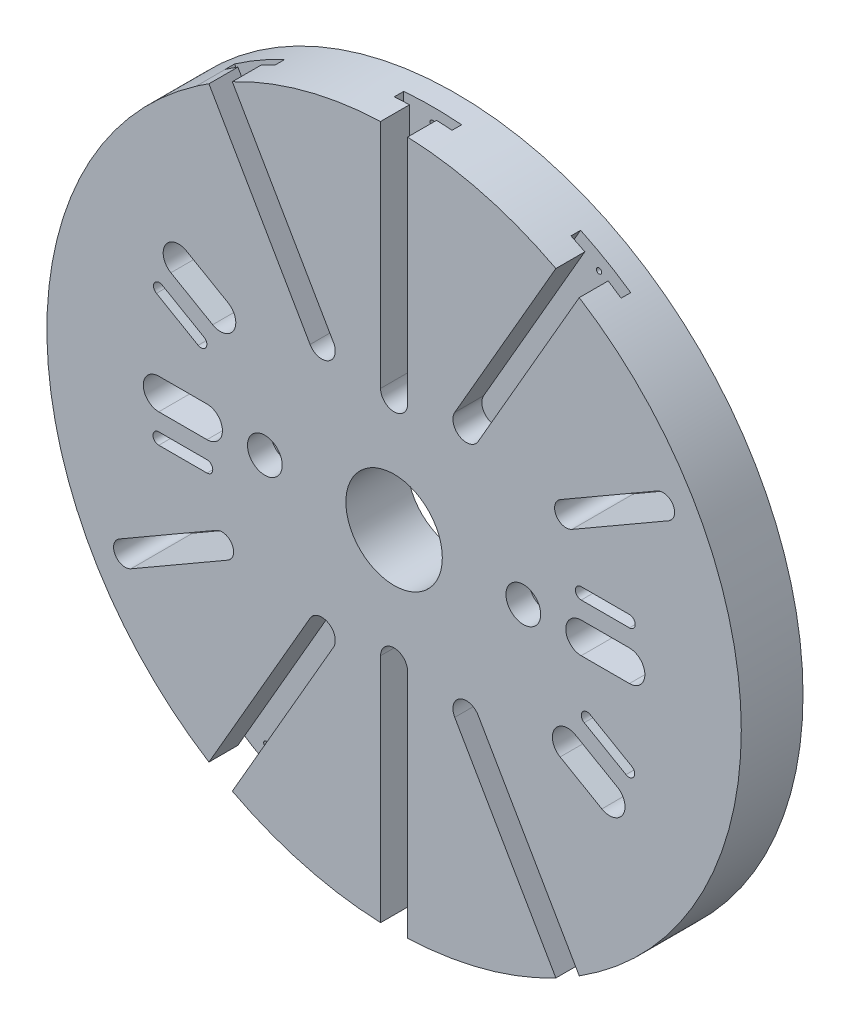
SolidWorks part; units mm, degrees
ref_plane "Front Plane" through (0, 0, 0) normal (0, 0, 1) x (1, 0, 0)
ref_plane "Top Plane" through (0, 0, 0) normal (0, 1, 0) x (1, 0, 0)
ref_plane "Right Plane" through (0, 0, 0) normal (1, 0, 0) x (0, 0, -1)
sketch "Sketch1" plane through (0, 0, 0) normal (0, 0, 1) x (1, 0, 0)
  circle A0 centre (0, 0) radius 180
  circle A1 centre (0, 0) radius 25
extrude "Boss-Extrude1" add sketch "Sketch1" along normal blind 32 contours A0 | A1
sketch "Sketch2" plane through (0, 0, 32) normal (0, 0, 1) x (1, 0, 0)
  line L0 (-198.9855, 0) -> (202.4357, 0) construction
  line L1 (0, 209.2415) -> (0, -209.2454) construction
  circle A0 centre (67, 0) radius 5.5
  circle A1 centre (-67, 0) radius 5.5
  dimension "D2" = 11
  dimension "D1" = 67
extrude "Cut-Extrude1" cut sketch "Sketch2" against normal through all
sketch "Sketch3" plane through (0, 0, 32) normal (0, 0, 1) x (1, 0, 0)
  line L1 (-86.2006, -56.6962) -> (-136.4301, -85.6962)
  line L3 (86.2006, 56.6962) -> (136.4301, 85.6962)
  line L4 (92.2006, 46.3038) -> (142.4301, 75.3038)
  line L5 (-92.2006, -46.3038) -> (-142.4301, -75.3038)
  arc A0 (86.2006, 56.6962) -> (92.2006, 46.3038) centre (89.2006, 51.5) ccw
  arc A1 (142.4301, 75.3038) -> (136.4301, 85.6962) centre (139.4301, 80.5) ccw
  arc A4 (-136.4301, -85.6962) -> (-142.4301, -75.3038) centre (-139.4301, -80.5) cw
  arc A5 (-92.2006, -46.3038) -> (-86.2006, -56.6962) centre (-89.2006, -51.5) cw
  dimension "D5" = 12
  dimension "D6" = 12
  dimension "D4" = 58
extrude "Cut-Extrude3" cut sketch "Sketch3" against normal through all contours L4 A1 L3 A0
ref_plane "Plane1" through (0, 0, 12) normal (0, 0, -1) x (-1, 0, 0)
sketch "Sketch5" plane through (0, 0, 12) normal (0, 0, -1) x (-1, 0, 0)
  line L1 (15, 60) -> (15, 264.0611)
  line L2 (-15, 60) -> (-15, 249.3757)
  line L3 (15, 264.0611) -> (-15, 249.3757)
  line L4 (-91.9564, 189.2731) -> (-117.9372, 174.2731)
  line L5 (-117.9372, 174.2731) -> (-50.4904, 57.4519)
  line L6 (-91.9564, 189.2731) -> (-24.5096, 72.4519)
  line L7 (91.9564, 189.2731) -> (24.5096, 72.4519)
  line L8 (117.9372, 174.2731) -> (50.4904, 57.4519)
  line L9 (91.9564, 189.2731) -> (117.9372, 174.2731)
  line L11 (91.9564, -189.2731) -> (117.9372, -174.2731)
  line L12 (117.9372, -174.2731) -> (50.4904, -57.4519)
  line L13 (91.9564, -189.2731) -> (24.5096, -72.4519)
  line L14 (-91.9564, -189.2731) -> (-24.5096, -72.4519)
  line L15 (-117.9372, -174.2731) -> (-50.4904, -57.4519)
  line L16 (-91.9564, -189.2731) -> (-117.9372, -174.2731)
  line L17 (10, -264.0611) -> (-15, -249.3757)
  line L18 (-15, -60) -> (-15, -249.3757)
  line L19 (15, -60) -> (10, -264.0611)
  arc A0 (-15, 60) -> (15, 60) centre (0, 60) ccw
  arc A2 (-50.4904, 57.4519) -> (-24.5096, 72.4519) centre (-37.5, 64.9519) ccw
  arc A3 (50.4904, 57.4519) -> (24.5096, 72.4519) centre (37.5, 64.9519) cw
  arc A4 (50.4904, -57.4519) -> (24.5096, -72.4519) centre (37.5, -64.9519) ccw
  arc A5 (-50.4904, -57.4519) -> (-24.5096, -72.4519) centre (-37.5, -64.9519) cw
  arc A6 (-15, -60) -> (15, -60) centre (0, -60) cw
  dimension "D1" = 15
  dimension "D3" = 15
  dimension "D4" = 15
  dimension "D2" = 15
  dimension "D5" = 15
  dimension "D6" = 15
extrude "Cut-Extrude4" cut sketch "Sketch5" against normal blind 5
sketch "Sketch6" plane through (0, 0, 32) normal (0, 0, 1) x (1, 0, 0)
  line L1 (-95.8846, -180.077) -> (-108.0089, -173.077)
  line L2 (-108.0089, -173.077) -> (-43.5622, -61.4519)
  line L3 (-31.4378, -68.4519) -> (-95.8846, -180.077)
  line L4 (-7, -254.4437) -> (-7, -60)
  line L5 (7, -245.6325) -> (-7, -254.4437)
  line L6 (7, -60) -> (7, -245.6325)
  line L7 (43.5622, -61.4519) -> (108.0089, -173.077)
  line L8 (95.8846, -180.077) -> (31.4378, -68.4519)
  line L9 (108.0089, 173.077) -> (95.8846, 180.077)
  line L10 (95.8846, 180.077) -> (31.4378, 68.4519)
  line L11 (43.5622, 61.4519) -> (108.0089, 173.077)
  line L12 (108.0089, -173.077) -> (95.8846, -180.077)
  line L18 (7, 60) -> (7, 245.6325)
  line L19 (7, 245.6325) -> (-7, 254.4437)
  line L20 (-7, 254.4437) -> (-7, 60)
  line L27 (-31.4378, 68.4519) -> (-95.8846, 180.077)
  line L28 (-108.0089, 173.077) -> (-43.5622, 61.4519)
  line L29 (-95.8846, 180.077) -> (-108.0089, 173.077)
  arc A0 (-43.5622, -61.4519) -> (-31.4378, -68.4519) centre (-37.5, -64.9519) cw
  arc A1 (-7, -60) -> (7, -60) centre (0, -60) cw
  arc A2 (31.4378, -68.4519) -> (43.5622, -61.4519) centre (37.5, -64.9519) cw
  arc A3 (31.4378, 68.4519) -> (43.5622, 61.4519) centre (37.5, 64.9519) ccw
  arc A6 (-7, 60) -> (7, 60) centre (0, 60) ccw
  arc A9 (-43.5622, 61.4519) -> (-31.4378, 68.4519) centre (-37.5, 64.9519) ccw
  dimension "D1" = 7
  dimension "D2" = 7
  dimension "D3" = 7
extrude "Cut-Extrude5" cut sketch "Sketch6" against normal up to next
sketch "Sketch7" plane through (0, 0, 32) normal (0, 0, 1) x (1, 0, 0)
  line L0 (0, 0) -> (0, 172.5) construction
  line L1 (0, 0) -> (86.25, 149.3894) construction
  circle A0 centre (0, 172.5) radius 1.375
  arc A1 (15, 179.3739) -> (-15, 179.3739) centre (0, 0) ccw construction
  circle A2 centre (86.25, 149.3894) radius 1.375
  circle A3 centre (149.3894, 86.25) radius 1.375 [skipped]
  circle A4 centre (172.5, 0) radius 1.375 [skipped]
  circle A5 centre (149.3894, -86.25) radius 1.375 [skipped]
  circle A6 centre (86.25, -149.3894) radius 1.375
  circle A7 centre (0, -172.5) radius 1.375
  circle A8 centre (-86.25, -149.3894) radius 1.375
  circle A9 centre (-149.3894, -86.25) radius 1.375 [skipped]
  circle A10 centre (-172.5, 0) radius 1.375 [skipped]
  circle A11 centre (-149.3894, 86.25) radius 1.375 [skipped]
  circle A12 centre (-86.25, 149.3894) radius 1.375
  point P2 (0, 180)
  dimension "D1" = 2.75
  dimension "D2" = 7.5
  dimension "D3" = 30
extrude "Cut-Extrude6" cut sketch "Sketch7" against normal through all
sketch "Sketch8" plane through (0, 0, 32) normal (0, 0, 1) x (1, 0, 0)
  line L0 (0, 0) -> (229.3619, 0) construction
  line L1 (97, 8) -> (122, 8)
  line L2 (97, -8) -> (122, -8)
  line L3 (97, 23) -> (122, 23)
  line L4 (0, 0) -> (181.224, -104.6297) construction
  line L5 (0, 0) -> (-183.3392, 105.8509) construction
  line L6 (120.2173, -49.7776) -> (98.5666, -37.2776)
  line L7 (122, 17) -> (97, 17)
  line L9 (41.5718, -88.0045) -> (54.0718, -109.6551) [skipped]
  line L10 (55.4282, -80.0045) -> (67.9282, -101.6551) [skipped]
  line L11 (75.7224, -97.1551) -> (63.2224, -75.5045) [skipped]
  line L12 (68.4186, -72.5045) -> (80.9186, -94.1551) [skipped]
  line L13 (-8, -97) -> (-8, -122) [skipped]
  line L14 (8, -97) -> (8, -122) [skipped]
  line L15 (17, -122) -> (17, -97) [skipped]
  line L16 (23, -97) -> (23, -122) [skipped]
  line L17 (-55.4282, -80.0045) -> (-67.9282, -101.6551) [skipped]
  line L18 (-41.5718, -88.0045) -> (-54.0718, -109.6551) [skipped]
  line L19 (-46.2776, -114.1551) -> (-33.7776, -92.5045) [skipped]
  line L20 (-28.5814, -95.5045) -> (-41.0814, -117.1551) [skipped]
  line L21 (-88.0045, -41.5718) -> (-109.6551, -54.0718) [skipped]
  line L22 (-80.0045, -55.4282) -> (-101.6551, -67.9282) [skipped]
  line L23 (-97.1551, -75.7224) -> (-75.5045, -63.2224) [skipped]
  line L24 (-72.5045, -68.4186) -> (-94.1551, -80.9186) [skipped]
  line L25 (-97, 8) -> (-122, 8)
  line L26 (-97, -8) -> (-122, -8)
  line L27 (-122, -17) -> (-97, -17)
  line L28 (-97, -23) -> (-122, -23)
  line L30 (86.0666, -58.9282) -> (107.7173, -71.4282)
  line L31 (94.0666, -45.0718) -> (115.7173, -57.5718)
  line L32 (101.5666, -32.0814) -> (123.2173, -44.5814)
  line L33 (-41.5718, 88.0045) -> (-54.0718, 109.6551) [skipped]
  line L34 (-55.4282, 80.0045) -> (-67.9282, 101.6551) [skipped]
  line L35 (-75.7224, 97.1551) -> (-63.2224, 75.5045) [skipped]
  line L36 (-68.4186, 72.5045) -> (-80.9186, 94.1551) [skipped]
  line L37 (8, 97) -> (8, 122) [skipped]
  line L38 (-8, 97) -> (-8, 122) [skipped]
  line L39 (-17, 122) -> (-17, 97) [skipped]
  line L40 (-23, 97) -> (-23, 122) [skipped]
  line L41 (55.4282, 80.0045) -> (67.9282, 101.6551) [skipped]
  line L42 (41.5718, 88.0045) -> (54.0718, 109.6551) [skipped]
  line L43 (46.2776, 114.1551) -> (33.7776, 92.5045) [skipped]
  line L44 (28.5814, 95.5045) -> (41.0814, 117.1551) [skipped]
  line L45 (88.0045, 41.5718) -> (109.6551, 54.0718) [skipped]
  line L46 (80.0045, 55.4282) -> (101.6551, 67.9282) [skipped]
  line L47 (97.1551, 75.7224) -> (75.5045, 63.2224) [skipped]
  line L48 (72.5045, 68.4186) -> (94.1551, 80.9186) [skipped]
  line L49 (-86.0666, 58.9282) -> (-107.7173, 71.4282)
  line L50 (-94.0666, 45.0718) -> (-115.7173, 57.5718)
  line L51 (-120.2173, 49.7776) -> (-98.5666, 37.2776)
  line L52 (-101.5666, 32.0814) -> (-123.2173, 44.5814)
  line L53 (-80.0045, 55.4282) -> (-101.6551, 67.9282) [skipped]
  line L54 (-88.0045, 41.5718) -> (-109.6551, 54.0718) [skipped]
  line L55 (-114.1551, 46.2776) -> (-92.5045, 33.7776) [skipped]
  line L56 (-95.5045, 28.5814) -> (-117.1551, 41.0814) [skipped]
  line L57 (80.0045, -55.4282) -> (101.6551, -67.9282) [skipped]
  line L58 (88.0045, -41.5718) -> (109.6551, -54.0718) [skipped]
  line L59 (114.1551, -46.2776) -> (92.5045, -33.7776) [skipped]
  line L60 (95.5045, -28.5814) -> (117.1551, -41.0814) [skipped]
  arc A0 (97, 8) -> (97, -8) centre (97, 0) ccw
  arc A1 (122, -8) -> (122, 8) centre (122, 0) ccw
  arc A4 (97, 23) -> (97, 17) centre (97, 20) ccw
  arc A5 (122, 17) -> (122, 23) centre (122, 20) ccw
  arc A6 (115.7173, -57.5718) -> (107.7173, -71.4282) centre (111.7173, -64.5) cw
  arc A7 (86.0666, -58.9282) -> (94.0666, -45.0718) centre (90.0666, -52) cw
  arc A8 (55.4282, -80.0045) -> (41.5718, -88.0045) centre (48.5, -84.0045) ccw [skipped]
  arc A9 (54.0718, -109.6551) -> (67.9282, -101.6551) centre (61, -105.6551) ccw [skipped]
  arc A10 (68.4186, -72.5045) -> (63.2224, -75.5045) centre (65.8205, -74.0045) ccw [skipped]
  arc A11 (75.7224, -97.1551) -> (80.9186, -94.1551) centre (78.3205, -95.6551) ccw [skipped]
  arc A12 (8, -97) -> (-8, -97) centre (0, -97) ccw [skipped]
  arc A13 (-8, -122) -> (8, -122) centre (0, -122) ccw [skipped]
  arc A14 (23, -97) -> (17, -97) centre (20, -97) ccw [skipped]
  arc A15 (17, -122) -> (23, -122) centre (20, -122) ccw [skipped]
  arc A16 (-41.5718, -88.0045) -> (-55.4282, -80.0045) centre (-48.5, -84.0045) ccw [skipped]
  arc A17 (-67.9282, -101.6551) -> (-54.0718, -109.6551) centre (-61, -105.6551) ccw [skipped]
  arc A18 (-28.5814, -95.5045) -> (-33.7776, -92.5045) centre (-31.1795, -94.0045) ccw [skipped]
  arc A19 (-46.2776, -114.1551) -> (-41.0814, -117.1551) centre (-43.6795, -115.6551) ccw [skipped]
  arc A20 (-80.0045, -55.4282) -> (-88.0045, -41.5718) centre (-84.0045, -48.5) ccw [skipped]
  arc A21 (-109.6551, -54.0718) -> (-101.6551, -67.9282) centre (-105.6551, -61) ccw [skipped]
  arc A22 (-72.5045, -68.4186) -> (-75.5045, -63.2224) centre (-74.0045, -65.8205) ccw [skipped]
  arc A23 (-97.1551, -75.7224) -> (-94.1551, -80.9186) centre (-95.6551, -78.3205) ccw [skipped]
  arc A24 (-97, -8) -> (-97, 8) centre (-97, 0) ccw
  arc A25 (-122, 8) -> (-122, -8) centre (-122, 0) ccw
  arc A26 (-97, -23) -> (-97, -17) centre (-97, -20) ccw
  arc A27 (-122, -17) -> (-122, -23) centre (-122, -20) ccw
  arc A28 (101.5666, -32.0814) -> (98.5666, -37.2776) centre (100.0666, -34.6795) ccw
  arc A29 (120.2173, -49.7776) -> (123.2173, -44.5814) centre (121.7173, -47.1795) ccw
  arc A32 (-55.4282, 80.0045) -> (-41.5718, 88.0045) centre (-48.5, 84.0045) ccw [skipped]
  arc A33 (-54.0718, 109.6551) -> (-67.9282, 101.6551) centre (-61, 105.6551) ccw [skipped]
  arc A34 (-68.4186, 72.5045) -> (-63.2224, 75.5045) centre (-65.8205, 74.0045) ccw [skipped]
  arc A35 (-75.7224, 97.1551) -> (-80.9186, 94.1551) centre (-78.3205, 95.6551) ccw [skipped]
  arc A36 (-8, 97) -> (8, 97) centre (0, 97) ccw [skipped]
  arc A37 (8, 122) -> (-8, 122) centre (0, 122) ccw [skipped]
  arc A38 (-23, 97) -> (-17, 97) centre (-20, 97) ccw [skipped]
  arc A39 (-17, 122) -> (-23, 122) centre (-20, 122) ccw [skipped]
  arc A40 (41.5718, 88.0045) -> (55.4282, 80.0045) centre (48.5, 84.0045) ccw [skipped]
  arc A41 (67.9282, 101.6551) -> (54.0718, 109.6551) centre (61, 105.6551) ccw [skipped]
  arc A42 (28.5814, 95.5045) -> (33.7776, 92.5045) centre (31.1795, 94.0045) ccw [skipped]
  arc A43 (46.2776, 114.1551) -> (41.0814, 117.1551) centre (43.6795, 115.6551) ccw [skipped]
  arc A44 (80.0045, 55.4282) -> (88.0045, 41.5718) centre (84.0045, 48.5) ccw [skipped]
  arc A45 (109.6551, 54.0718) -> (101.6551, 67.9282) centre (105.6551, 61) ccw [skipped]
  arc A46 (72.5045, 68.4186) -> (75.5045, 63.2224) centre (74.0045, 65.8205) ccw [skipped]
  arc A47 (97.1551, 75.7224) -> (94.1551, 80.9186) centre (95.6551, 78.3205) ccw [skipped]
  arc A48 (-94.0666, 45.0718) -> (-86.0666, 58.9282) centre (-90.0666, 52) ccw
  arc A49 (-107.7173, 71.4282) -> (-115.7173, 57.5718) centre (-111.7173, 64.5) ccw
  arc A50 (-101.5666, 32.0814) -> (-98.5666, 37.2776) centre (-100.0666, 34.6795) ccw
  arc A51 (-120.2173, 49.7776) -> (-123.2173, 44.5814) centre (-121.7173, 47.1795) ccw
  arc A52 (-88.0045, 41.5718) -> (-80.0045, 55.4282) centre (-84.0045, 48.5) ccw [skipped]
  arc A53 (-101.6551, 67.9282) -> (-109.6551, 54.0718) centre (-105.6551, 61) ccw [skipped]
  arc A54 (-95.5045, 28.5814) -> (-92.5045, 33.7776) centre (-94.0045, 31.1795) ccw [skipped]
  arc A55 (-114.1551, 46.2776) -> (-117.1551, 41.0814) centre (-115.6551, 43.6795) ccw [skipped]
  arc A56 (101.6551, -67.9282) -> (109.6551, -54.0718) centre (105.6551, -61) ccw [skipped]
  arc A57 (95.5045, -28.5814) -> (92.5045, -33.7776) centre (94.0045, -31.1795) ccw [skipped]
  arc A58 (114.1551, -46.2776) -> (117.1551, -41.0814) centre (115.6551, -43.6795) ccw [skipped]
  arc A59 (88.0045, -41.5718) -> (80.0045, -55.4282) centre (84.0045, -48.5) ccw [skipped]
  point P150 (0, 0)
  dimension "D1" = 25
  dimension "D3" = 30
  dimension "D5" = 8
  dimension "D8" = 3
  dimension "D13" = 8
  dimension "D14" = 3
  dimension "D2" = 97
  dimension "D4" = 150
  dimension "D6" = 25
  dimension "D7" = 104
  dimension "D9" = 25
  dimension "D11" = 20
  dimension "D12" = 12
extrude "Cut-Extrude7" cut sketch "Sketch8" against normal blind 17.2
sketch "Sketch9" plane through (0, 0, 32) normal (0, 0, 1) x (1, 0, 0)
  line L0 (-104.2173, 77.4904) -> (-82.5666, 64.9904)
  line L1 (-122, 15) -> (-97, 15)
  line L2 (-119.2173, 51.5096) -> (-97.5666, 39.0096)
  line L4 (-97, -15) -> (-122, -15)
  line L5 (97, -15) -> (122, -15)
  line L6 (122, 15) -> (97, 15)
  line L8 (104.2173, -77.4904) -> (82.5666, -64.9904)
  line L9 (119.2173, -51.5096) -> (97.5666, -39.0096)
  arc A0 (-122, 15) -> (-122, -15) centre (-122, 0) ccw
  arc A1 (-104.2173, 77.4904) -> (-119.2173, 51.5096) centre (-111.7173, 64.5) ccw
  arc A2 (-97, -15) -> (-97, 15) centre (-97, 0) ccw
  arc A3 (-97.5666, 39.0096) -> (-82.5666, 64.9904) centre (-90.0666, 52) ccw
  arc A4 (97, -15) -> (97, 15) centre (97, 0) cw
  arc A5 (122, 15) -> (122, -15) centre (122, 0) cw
  arc A6 (82.5666, -64.9904) -> (97.5666, -39.0096) centre (90.0666, -52) cw
  arc A7 (119.2173, -51.5096) -> (104.2173, -77.4904) centre (111.7173, -64.5) cw
extrude "Cut-Extrude8" cut sketch "Sketch9" along normal blind 15 from surface at -32 starting at face at (-84.875, 149.3894, 0)
sketch "Sketch10" plane through (0, 0, 32) normal (0, 0, 1) x (1, 0, 0)
  line L0 (111.7173, -64.5) -> (90.0666, -52)
  line L1 (-90.0666, 52) -> (-111.7173, 64.5)
  line L2 (-100.0666, 34.6795) -> (-121.7173, 47.1795)
  line L3 (121.7173, -47.1795) -> (100.0666, -34.6795)
ref_plane "Plane2" through (0, 0, 0) normal (-0.5, -0.866, 0) x (-0.866, 0.5, 0)
sketch "Sketch11" plane through (0, 0, 32) normal (0, 0, 1) x (1, 0, 0)
  circle A0 centre (-67, 0) radius 9
  circle A1 centre (67, 0) radius 9
extrude "Cut-Extrude9" cut sketch "Sketch11" against normal blind 12
sketch "Sketch12" plane through (0, 0, 0) normal (0, 0, -1) x (-1, 0, 0)
  circle A1 centre (-33.5, -58.0237) radius 5.5
  circle A3 centre (33.5, 58.0237) radius 5.5
extrude "Cut-Extrude10" cut sketch "Sketch12" against normal blind 11
